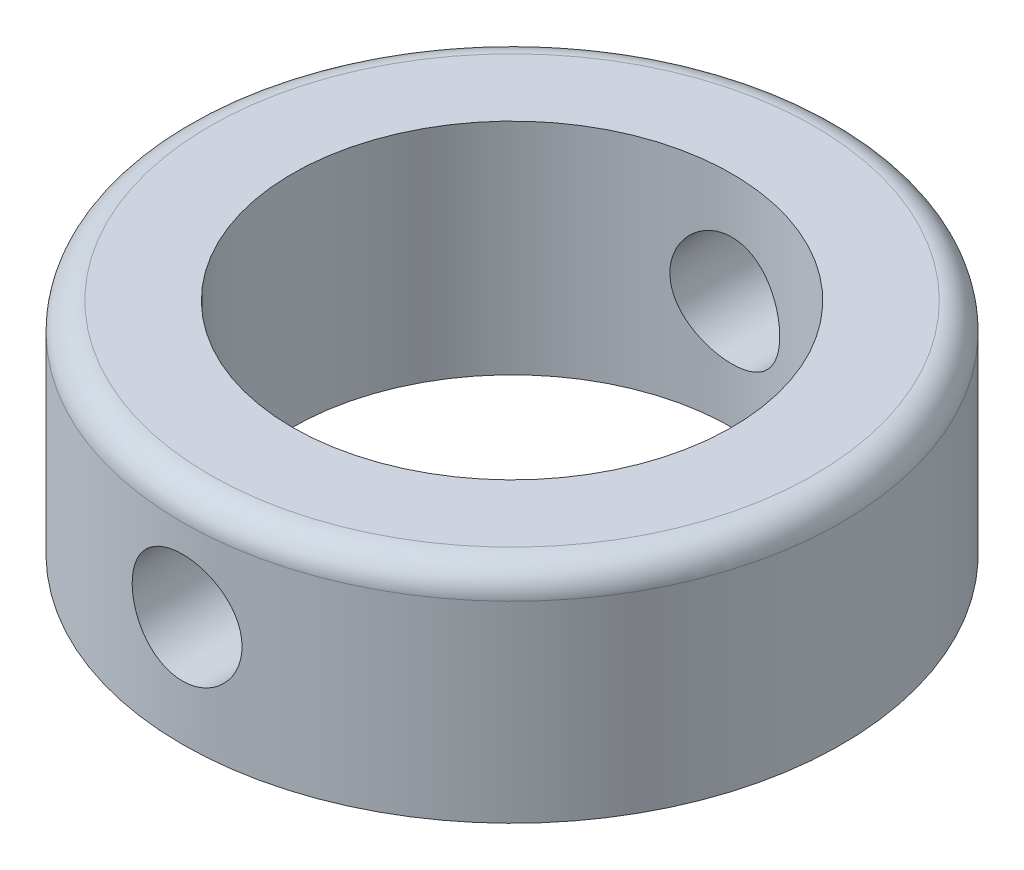
from build123d import *

# Parameters (mm, degrees)
SKETCH1_R               = 12
SKETCH1_R_2             = 8
BOSS_EXTRUDE1_DEPTH     = 8
CUT_EXTRUDE1_DEPTH      = 19.761663039
CUT_EXTRUDE1_DEPTH_BACK = 19.761663039
SKETCH2_R               = 2
FILLET1_R               = 1


with BuildPart() as part:
    # Sketch1 → Boss-Extrude1 (new body)
    with BuildSketch(Plane(origin=(0, 0, 0), x_dir=(1, 0, 0), z_dir=(0, 1, 0))):
        with Locations(Location((0, 0, 0), (0, 0, 270))):
            Circle(SKETCH1_R)
        with Locations(Location((0, 0, 0), (0, 0, 270))):
            Circle(SKETCH1_R_2, mode=Mode.SUBTRACT)
    extrude(amount=-BOSS_EXTRUDE1_DEPTH)

    # Sketch2 → Cut-Extrude1 (cut, two sides: drawn at the far end of the back side and taken through both)
    with BuildSketch(Plane.XY.offset(-CUT_EXTRUDE1_DEPTH_BACK)):
        with Locations((0, -4)):
            Circle(SKETCH2_R)
    extrude(amount=CUT_EXTRUDE1_DEPTH + CUT_EXTRUDE1_DEPTH_BACK, mode=Mode.SUBTRACT)

    # Fillet1
    fillet1_edges = [part.edges().sort_by_distance(p)[0] for p in [
        (0, 0, -12),
    ]]
    fillet(fillet1_edges, radius=FILLET1_R)


solid = part.part
